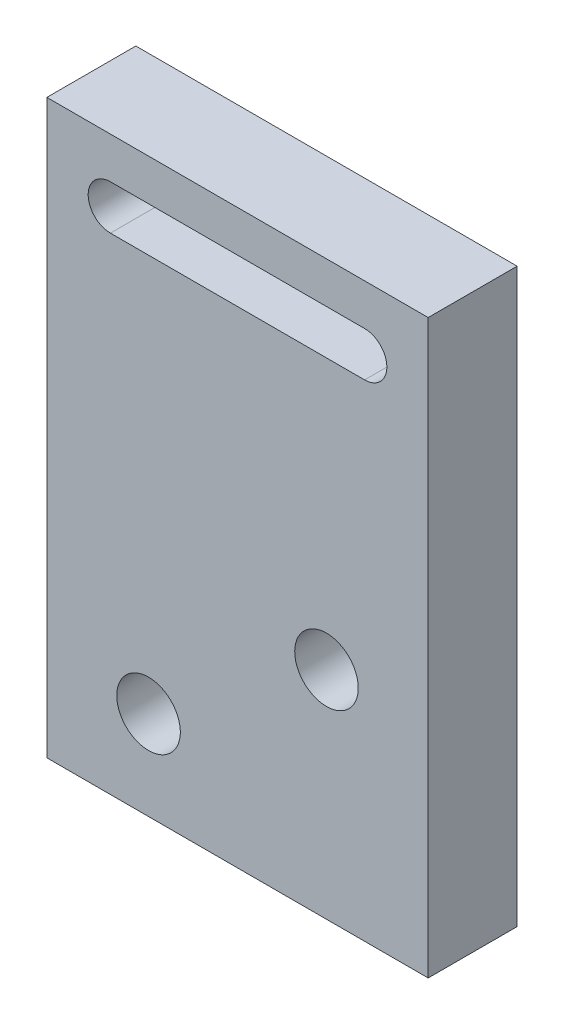
SolidWorks part; units mm, degrees
ref_plane "Front Plane" through (0, 0, 0) normal (0, 0, 1) x (1, 0, 0)
ref_plane "Top Plane" through (0, 0, 0) normal (0, 1, 0) x (1, 0, 0)
ref_plane "Right Plane" through (0, 0, 0) normal (1, 0, 0) x (0, 0, -1)
sketch "Sketch 1" plane through (0, 0, 0) normal (0, 0, 1) x (1, 0, 0)
  line L1 (-15, -22.5) -> (15, -22.5)
  line L2 (-15, -22.5) -> (-15, 22.5)
  line L3 (-15, 22.5) -> (15, 22.5)
  line L4 (15, -22.5) -> (15, 22.5)
  line L5 (-15, -22.5) -> (15, 22.5) construction
  line L6 (-15, 22.5) -> (15, -22.5) construction
  point P0 (0, 0)
  dimension "D1" = 45
  dimension "D2" = 30
extrude "Boss-Extrude 1" add sketch "Sketch 1" along normal blind 7
sketch "Sketch 2" plane through (0, 0, 0) normal (0, 0, -1) x (-1, 0, 0)
  line L0 (10, 17.5) -> (-10, 17.5) construction
  line L1 (10, 15.75) -> (-10, 15.75)
  line L2 (10, 19.25) -> (-10, 19.25)
  line L3 (-15, -22.5) -> (-15, 22.5) construction
  line L4 (-15, 22.5) -> (15, 22.5) construction
  arc A0 (10, 15.75) -> (10, 19.25) centre (10, 17.5) ccw
  arc A1 (-10, 19.25) -> (-10, 15.75) centre (-10, 17.5) ccw
  point P2 (0, 17.5)
  dimension "D1" = 3.5
  dimension "D2" = 20
  dimension "D3" = 15
  dimension "D4" = 5
extrude "Cut-Extrude 1" cut sketch "Sketch 2" against normal through all
hole_wizard "M6 Tapped Hole 1" positions "Sketch 4" profile "Sketch 3" tap size "M6" standard "GB" end condition through all
sketch "Sketch 4" plane through (0, 0, 0) normal (0, 0, -1) x (-1, 0, 0)
  line L0 (15, 22.5) -> (15, -22.5) construction
  line L1 (15, -22.5) -> (-15, -22.5) construction
  point P0 (7, -15.5)
  point P8 (-7, -5.5)
  dimension "D1" = 8
  dimension "D2" = 7
  dimension "D3" = 10
  dimension "D4" = 14
sketch "Sketch 3" plane through (-7, -15.5, 0) normal (1, 0, 0) x (0, 1, 0)
  line L0 (0, 0) -> (0, 7)
  line L1 (0, 7) -> (2.5, 7)
  line L2 (2.5, 7) -> (2.5, 0)
  line L5 (2.5, 0) -> (0, 0)
  line L11 (0, -6.35) -> (0, 107.95) construction
  dimension "貫穿螺孔鑽直徑" = 5
  dimension "貫穿螺孔鑽深度" = 7
cosmetic thread "Cosmetic Thread 1" parameters "D2"=6
cosmetic thread "Cosmetic Thread 2" parameters "D2"=6
